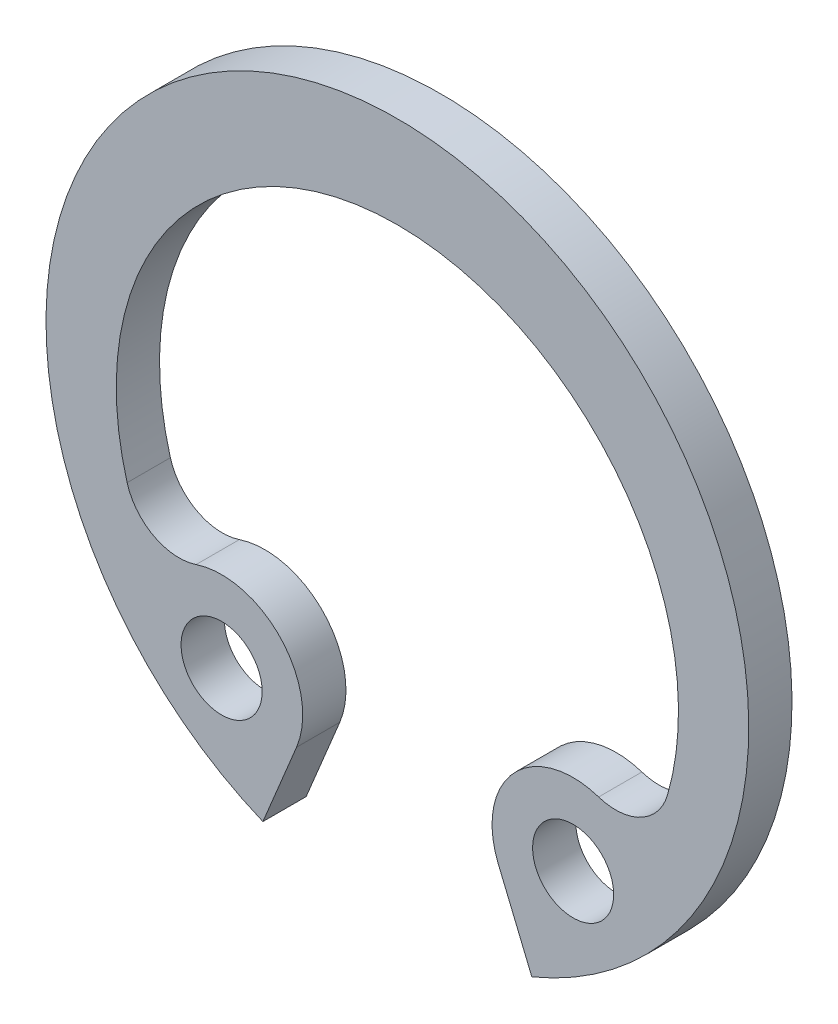
SolidWorks part; units mm, degrees
ref_plane "Front" through (0, 0, 0) normal (0, 0, 1) x (1, 0, 0)
ref_plane "Top" through (0, 0, 0) normal (0, 1, 0) x (1, 0, 0)
ref_plane "Right" through (0, 0, 0) normal (1, 0, 0) x (0, 0, -1)
sketch "Sketch1" plane through (0, 0, 0) normal (0, 0, 1) x (1, 0, 0)
  line L0 (0, 0) -> (-1.8654, -4.5034) construction
  line L1 (0, 7.3554) -> (0, -7.1505) construction
  line L2 (1.8654, -4.5034) -> (2.4874, -6.0052)
  line L4 (-1.8654, -4.5034) -> (-2.4874, -6.0052)
  arc A0 (2.4874, -6.0052) -> (-2.4874, -6.0052) centre (0, 0) ccw
  arc A1 (4.999, -1.8316) -> (-4.999, -1.8316) centre (0, -0.4) ccw
  arc A2 (-1.8654, -4.5034) -> (-3.7231, -2.5055) centre (-3.2512, -3.9294) ccw
  arc A3 (-4.999, -1.8316) -> (-3.7231, -2.5055) centre (-4.0377, -1.5563) ccw
  circle A4 centre (3.2512, -3.9294) radius 0.75
  arc A5 (4.999, -1.8316) -> (3.7231, -2.5055) centre (4.0377, -1.5563) cw
  arc A6 (-5.1, 0) -> (5.1, 0) centre (0, 0) ccw construction
  circle A7 centre (-3.2512, -3.9294) radius 0.75
  arc A8 (1.8654, -4.5034) -> (3.7231, -2.5055) centre (3.2512, -3.9294) cw
  dimension "D" = 13
  dimension "d0" = 10.4
  dimension "R1" = 1.5
  dimension "R2" = 1
  dimension "d1" = 1.5
  dimension "R" = 5.1
  dimension "C" = 0.4
  dimension "Angle" = 45
extrude "Body" add sketch "Sketch1" against normal blind 0.8
